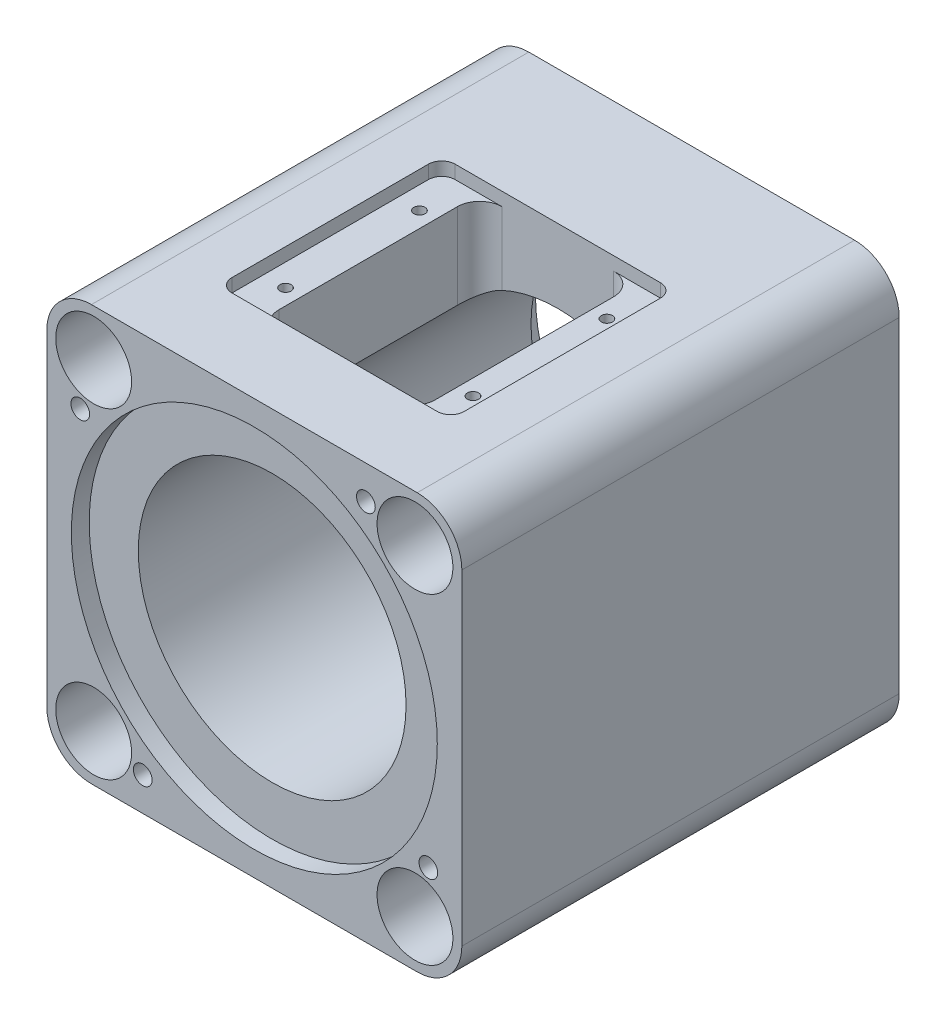
SolidWorks part; units mm, degrees
ref_plane "Front Plane" through (0, 0, 0) normal (0, 0, 1) x (1, 0, 0)
ref_plane "Top Plane" through (0, 0, 0) normal (0, 1, 0) x (1, 0, 0)
ref_plane "Right Plane" through (0, 0, 0) normal (1, 0, 0) x (0, 0, -1)
sketch "Sketch1" plane through (0, 0, 0) normal (0, 0, 1) x (1, 0, 0)
  line L1 (-46.5, -46.5) -> (46.5, -46.5)
  line L2 (-46.5, -46.5) -> (-46.5, 46.5)
  line L3 (-46.5, 46.5) -> (46.5, 46.5)
  line L4 (46.5, -46.5) -> (46.5, 46.5)
  line L5 (-46.5, -46.5) -> (46.5, 46.5) construction
  line L6 (-46.5, 46.5) -> (46.5, -46.5) construction
  point P0 (0, 0)
  dimension "D1" = 93
  dimension "D2" = 93
extrude "Boss-Extrude1" add sketch "Sketch1" along normal blind 98
sketch "Sketch2" plane through (0, 0, 0) normal (0, 0, -1) x (-1, 0, 0)
  circle A0 centre (0, 0) radius 35
  dimension "D1" = 70
extrude "Cut-Extrude1" cut sketch "Sketch2" against normal blind 6
sketch "Sketch3" plane through (0, 0, 6) normal (0, 0, -1) x (-1, 0, 0)
  circle A0 centre (0, 0) radius 30
  dimension "D1" = 60
extrude "Cut-Extrude2" cut sketch "Sketch3" against normal through all
sketch "Sketch4" plane through (0, 46.5, 0) normal (0, 1, 0) x (1, 0, 0)
  line L0 (0, 0) -> (0, -30) construction
  line L1 (17.5, -30) -> (-17.5, -30)
  line L2 (17.5, -30) -> (17.5, -80)
  line L3 (17.5, -80) -> (-17.5, -80)
  line L4 (-17.5, -30) -> (-17.5, -80)
  line L5 (46.5, 0) -> (-46.5, 0) construction
  dimension "D1" = 35
  dimension "D2" = 50
  dimension "D3" = 30
extrude "Cut-Extrude3" cut sketch "Sketch4" against normal up to surface (46.5 mm away) up to plane "Top Plane"
fillet "Fillet1" radius 10 4 edges at (-46.5, -46.5, 49) (46.5, -46.5, 49) (46.5, 46.5, 49) (-46.5, 46.5, 49)
hole_wizard "CBORE for M10 Hex Head Bolt1" positions "Sketch5" profile "Sketch6" counterbore size "M10" standard "GB" end condition through all
sketch "Sketch5" plane through (0, 0, 98) normal (0, 0, 1) x (1, 0, 0)
  line L0 (0, 0) -> (0, 30)
  line L1 (0, 0) -> (-30, 0)
  circle A1 centre (0, 0) radius 30 construction
  point P0 (-36, 36)
  point P14 (36, 36)
  point P15 (36, -36)
  point P16 (-36, -36)
  dimension "D1" = 72
  dimension "D2" = 72
sketch "Sketch6" plane through (-36, 36, 98) normal (1, 0, 0) x (0, -1, 0)
  line L0 (0, 0) -> (0, 98)
  line L1 (0, 98) -> (5.5, 98)
  line L3 (5.5, 98) -> (5.5, 78)
  line L4 (5.5, 78) -> (8.5, 78)
  line L5 (8.5, 78) -> (8.5, 0)
  line L7 (8.5, 0) -> (0, 0)
  line L11 (0, -6.35) -> (0, 107.95) construction
  dimension "通孔孔直径" = 11
  dimension "通孔孔深度" = 98
  dimension "柱形沉头孔直径" = 17
  dimension "柱形沉头孔深度" = 78
sketch "Sketch9" plane through (0, 0, 98) normal (0, 0, 1) x (1, 0, 0)
  circle A0 centre (0, 0) radius 41
  dimension "D1" = 82
extrude "Cut-Extrude4" cut sketch "Sketch9" against normal blind 4
sketch "Sketch10" plane through (0, 46.5, 0) normal (0, 1, 0) x (1, 0, 0)
  line L4 (17.5, -30) -> (-17.5, -30) construction
  line L5 (26, -30) -> (-26, -30)
  line L6 (26, -30) -> (26, -80)
  line L7 (26, -80) -> (-26, -80)
  line L8 (-26, -30) -> (-26, -80)
  line L9 (-17.5, -80) -> (17.5, -80) construction
  line L10 (17.5, -55) -> (26, -55) construction
  line L11 (17.5, -80) -> (17.5, -30) construction
  line L16 (-17.5, -55) -> (-26, -55) construction
  line L17 (-17.5, -30) -> (-17.5, -80) construction
  dimension "D1" = 52
extrude "Cut-Extrude5" cut sketch "Sketch10" against normal blind 3
fillet "Fillet2" radius 3 4 edges at (-26, 45, 30) (-26, 45, 80) (26, 45, 80) (26, 45, 30)
hole_wizard "M3 Tapped Hole1" positions "Sketch11" profile "Sketch12" tap size "M3" standard "GB"
sketch "Sketch11" plane through (0, 43.5, 0) normal (0, 1, 0) x (1, 0, 0)
  line L0 (-17.5, -55) -> (17.5, -55)
  line L1 (-17.5, -30) -> (-17.5, -80) construction
  line L2 (17.5, -80) -> (17.5, -30) construction
  line L3 (0, -30) -> (0, -55)
  line L4 (23, -30) -> (-23, -30) construction
  point P0 (21, -40)
  point P14 (21, -70)
  point P15 (-21, -70)
  point P16 (-21, -40)
  dimension "D1" = 42
  dimension "D2" = 30
sketch "Sketch12" plane through (21, 43.5, 40) normal (1, 0, 0) x (0, 0, 1)
  line L0 (0, 0) -> (0, 8.2511)
  line L1 (0, 8.2511) -> (1.25, 7.5)
  line L2 (1.25, 7.5) -> (1.25, 0)
  line L5 (1.25, 0) -> (0, 0)
  line L10 (0, 8.2511) -> (-1.25, 7.5) construction
  line L11 (0, -6.35) -> (0, 107.95) construction
  dimension "螺纹孔钻头直径" = 2.5
  dimension "螺纹孔钻头深度" = 7.5
  dimension "导头角度" = 118
cosmetic thread "Cosmetic Thread 5" parameters "D1"=6, "D2"=3
cosmetic thread "Cosmetic Thread 6" parameters "D1"=6, "D2"=3
cosmetic thread "Cosmetic Thread 7" parameters "D1"=6, "D2"=3
cosmetic thread "Cosmetic Thread 8" parameters "D1"=6, "D2"=3
hole_wizard "M5 Tapped Hole1" positions "Sketch7" profile "Sketch8" tap size "M5" standard "GB"
sketch "Sketch7" plane through (0, 0, 94) normal (0, 0, 1) x (1, 0, 0)
  line L0 (0, 0) -> (0, 32.5)
  line L1 (0, 0) -> (-32.5, 0)
  circle A0 centre (0, 0) radius 32.5
  point P0 (0, 32.5)
  point P15 (-32.5, 0)
  point P17 (0, -32.5)
  point P21 (32.5, 0)
  dimension "D1" = 65
sketch "Sketch8" plane through (0, 32.5, 94) normal (1, 0, 0) x (0, -1, 0)
  line L0 (0, 0) -> (0, 11.2618)
  line L1 (0, 11.2618) -> (2.1, 10)
  line L2 (2.1, 10) -> (2.1, 0)
  line L5 (2.1, 0) -> (0, 0)
  line L10 (0, 11.2618) -> (-2.1, 10) construction
  line L11 (0, -6.35) -> (0, 107.95) construction
  dimension "螺纹孔钻头直径" = 4.2
  dimension "螺纹孔钻头深度" = 10
  dimension "导头角度" = 118
cosmetic thread "Cosmetic Thread 1" [suppressed] parameters "D1"=10, "D2"=5
cosmetic thread "Cosmetic Thread 2" [suppressed] parameters "D1"=10, "D2"=5
cosmetic thread "Cosmetic Thread 3" [suppressed] parameters "D1"=10, "D2"=5
cosmetic thread "Cosmetic Thread 4" [suppressed] parameters "D1"=10, "D2"=5
fillet "Fillet3" radius 5 4 edges at (17.5, 33.9335, 30) (-17.5, 33.9335, 30) (-17.5, 33.9335, 80) (17.5, 33.9335, 80)
hole_wizard "M5 Tapped Hole2" positions "Sketch13" profile "Sketch14" tap size "M5" standard "GB"
sketch "Sketch13" plane through (0, 0, 98) normal (0, 0, 1) x (1, 0, 0)
  line L0 (46.5, -36.5) -> (46.5, 36.5) construction
  line L1 (36.5, 46.5) -> (-36.5, 46.5) construction
  point P0 (25, 39)
  dimension "D1" = 21.5
  dimension "D2" = 7.5
sketch "Sketch14" plane through (25, 39, 98) normal (1, 0, 0) x (0, -1, 0)
  line L0 (0, 0) -> (0, 13.6618)
  line L1 (0, 13.6618) -> (2.1, 12.4)
  line L2 (2.1, 12.4) -> (2.1, 0)
  line L5 (2.1, 0) -> (0, 0)
  line L10 (0, 13.6618) -> (-2.1, 12.4) construction
  line L11 (0, -6.35) -> (0, 107.95) construction
  dimension "螺纹孔钻头直径" = 4.2
  dimension "螺纹孔钻头深度" = 12.4
  dimension "导头角度" = 118
cosmetic thread "Cosmetic Thread 9" parameters "D1"=10, "D2"=5
pattern_circular "CirPattern1" count 4 every 90 about axis through (0, 0, 0) along (0, 0, 1) of "M5 Tapped Hole2"
